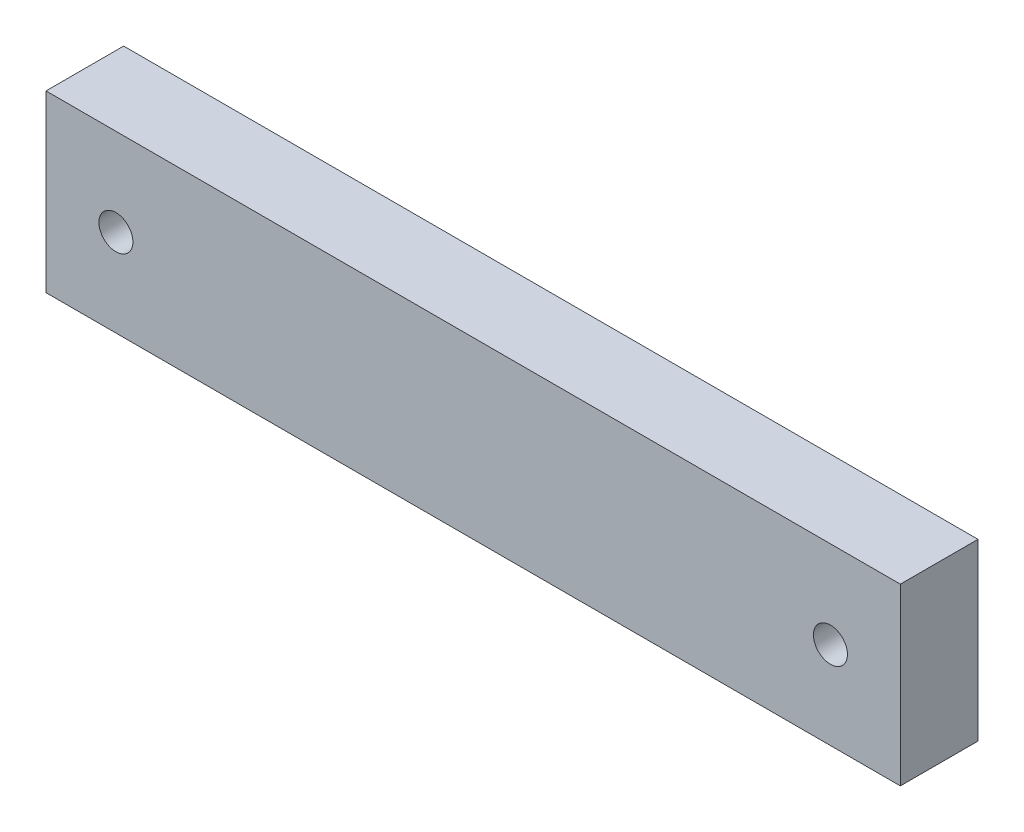
SolidWorks part; units mm, degrees
ref_plane "Front Plane" through (0, 0, 0) normal (0, 0, 1) x (1, 0, 0)
ref_plane "Top Plane" through (0, 0, 0) normal (0, 1, 0) x (1, 0, 0)
ref_plane "Right Plane" through (0, 0, 0) normal (1, 0, 0) x (0, 0, -1)
sketch "Sketch1" plane through (0, 0, 0) normal (0, 0, 1) x (1, 0, 0)
  line L0 (0, 45) -> (440, 45) construction
  line L1 (0, 0) -> (440, 0)
  line L2 (0, 0) -> (0, 90)
  line L3 (0, 90) -> (440, 90)
  line L4 (440, 0) -> (440, 90)
  dimension "D1" = 90
  dimension "D2" = 440
extrude "Boss-Extrude1" add sketch "Sketch1" along normal blind 40
hole_wizard "M20 Tapped Hole1" positions "Sketch3" profile "Sketch2" tap size "M20" standard "GB" end condition through all
sketch "Sketch3" plane through (0, 0, 40) normal (0, 0, 1) x (1, 0, 0)
  line L0 (0, 45) -> (440, 45) construction
  line L1 (0, 90) -> (0, 0) construction
  line L2 (440, 0) -> (440, 90) construction
  point P0 (36, 45)
  point P1 (404, 45)
  dimension "D1" = 36
  dimension "D2" = 368
sketch "Sketch2" plane through (36, 45, 40) normal (1, 0, 0) x (0, -1, 0)
  line L0 (0, 0) -> (0, 40)
  line L1 (0, 40) -> (8.75, 40)
  line L2 (8.75, 40) -> (8.75, 0)
  line L5 (8.75, 0) -> (0, 0)
  line L11 (0, -6.35) -> (0, 107.95) construction
  dimension "通孔螺纹孔钻头直径" = 17.5
  dimension "通孔螺纹孔钻头深度" = 40
cosmetic thread "Cosmetic Thread 1"
cosmetic thread "Cosmetic Thread 2"
